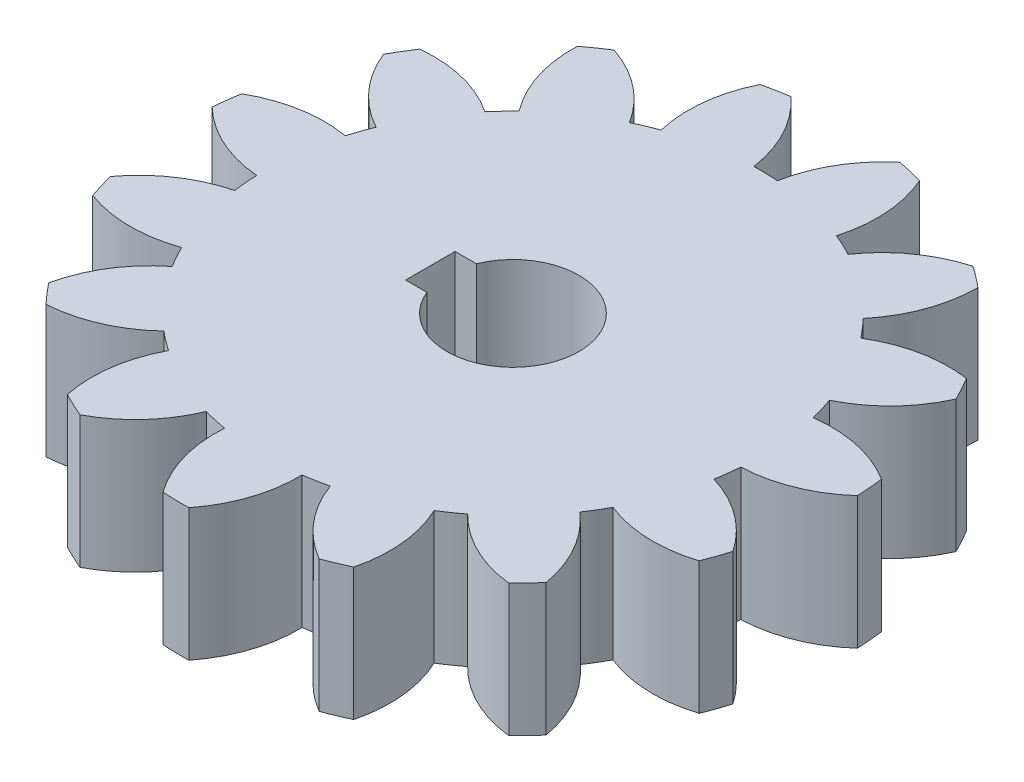
SolidWorks part; units mm, degrees
ref_plane "Front Plane" through (0, 0, 0) normal (0, 0, 1) x (1, 0, 0)
ref_plane "Top Plane" through (0, 0, 0) normal (0, 1, 0) x (1, 0, 0)
ref_plane "Right Plane" through (0, 0, 0) normal (1, 0, 0) x (0, 0, -1)
other "Configuration Table"
sketch "Sketch1" plane through (0, 0, 0) normal (0, 1, 0) x (1, 0, 0)
  line L0 (-43.1275, 149.2664) -> (-24.4163, 51.0325) construction
  line L1 (-42.9568, 58.5325) -> (-49.4163, 58.5325)
  line L2 (-42.9568, 43.5325) -> (-49.4163, 43.5325)
  line L5 (-49.4163, 43.5325) -> (-49.4163, 58.5325)
  line L6 (5.1882, 42.1512) -> (-49.4163, 58.5325) construction
  line L7 (5.1882, 59.9139) -> (-49.4163, 43.5325) construction
  arc A0 (-47.0419, 148.4393) -> (-39.1832, 149.9362) centre (-24.4163, 51.0325) cw
  arc A1 (10.8043, 117.2482) -> (4.1913, 120.3622) centre (-24.4163, 51.0325) ccw
  arc A2 (-47.0419, 148.4393) -> (-50.057, 121.5134) centre (-11.1471, 130.7882) ccw
  arc A3 (-39.1832, 149.9362) -> (-26.4808, 126.0041) centre (-66.0757, 120.3256) cw
  arc A4 (-5.4669, 149.2207) -> (-19.173, 125.849) centre (20.1453, 118.4959) ccw
  arc A5 (2.3213, 147.3918) -> (4.1913, 120.3622) centre (-34.29, 131.2793) cw
  arc A6 (-5.4669, 149.2207) -> (2.3213, 147.3918) centre (-24.4163, 51.0325) cw
  arc A7 (32.8316, 133.0245) -> (10.8043, 117.2482) centre (43.7325, 94.5385) ccw
  arc A8 (39.2025, 128.186) -> (29.917, 102.7326) centre (-0.7971, 128.3576) cw
  arc A9 (32.8316, 133.0245) -> (39.2025, 128.186) centre (-24.4163, 51.0325) cw
  arc A10 (61.2314, 102.6511) -> (34.6916, 97.1981) centre (55.5362, 63.0586) ccw
  arc A11 (65.0835, 95.6396) -> (46.2479, 76.1635) centre (28.6118, 112.0657) cw
  arc A12 (61.2314, 102.6511) -> (65.0835, 95.6396) centre (-24.4163, 51.0325) cw
  arc A13 (74.8219, 63.3524) -> (48.3587, 69.1655) centre (53.5154, 29.4993) ccw
  arc A14 (75.4892, 55.3803) -> (50.3604, 45.2491) centre (48.8517, 85.2207) cw
  arc A15 (74.8219, 63.3524) -> (75.4892, 55.3803) centre (-24.4163, 51.0325) cw
  arc A16 (71.2533, 21.9235) -> (49.4423, 37.9976) centre (38.0195, -0.3367) ccw
  arc A17 (68.6203, 14.3692) -> (41.5433, 15.3347) centre (56.423, 52.4642) cw
  arc A18 (71.2533, 21.9235) -> (68.6203, 14.3692) centre (-24.4163, 51.0325) cw
  arc A19 (51.1425, -14.4722) -> (37.7551, 9.0835) centre (11.7279, -21.2906) ccw
  arc A20 (45.6645, -20.3025) -> (21.3212, -8.4072) centre (50.0163, 19.4601) cw
  arc A21 (51.1425, -14.4722) -> (45.6645, -20.3025) centre (-24.4163, 51.0325) cw
  arc A22 (17.9669, -39.5415) -> (15.3179, -12.5772) centre (-20.8134, -29.7391) ccw
  arc A23 (10.5911, -42.6397) -> (-6.8094, -21.8715) centre (30.7396, -8.0848) cw
  arc A24 (17.9669, -39.5415) -> (10.5911, -42.6397) centre (-24.4163, 51.0325) cw
  arc A25 (-22.5371, -48.9498) -> (-13.9897, -23.2392) centre (-53.9777, -24.2214) ccw
  arc A26 (-30.5353, -48.7801) -> (-37.9843, -22.73) centre (1.926, -25.4077) cw
  arc A27 (-22.5371, -48.9498) -> (-30.5353, -48.7801) centre (-24.4163, 51.0325) cw
  arc A28 (-63.3661, -41.0702) -> (-45.1002, -21.0589) centre (-82.0305, -5.6917) ccw
  arc A29 (-70.6038, -37.662) -> (-66.8132, -10.8343) centre (-31.4425, -29.5135) cw
  arc A30 (-63.3661, -41.0702) -> (-70.6038, -37.662) centre (-24.4163, 51.0325) cw
  arc A31 (-97.4602, -17.2652) -> (-72.6342, -6.4134) centre (-100.1213, 22.6462) ccw
  arc A32 (-102.6859, -11.2078) -> (-88.3113, 11.7588) centre (-63.5961, -19.6921) cw
  arc A33 (-97.4602, -17.2652) -> (-102.6859, -11.2078) centre (-24.4163, 51.0325) cw
  arc A34 (-118.9244, 18.3491) -> (-91.8309, 18.1651) centre (-105.122, 55.8923) ccw
  arc A35 (-121.2346, 26.0083) -> (-98.7614, 41.1426) centre (-88.9751, 2.3582) cw
  arc A36 (-118.9244, 18.3491) -> (-121.2346, 26.0083) centre (-24.4163, 51.0325) cw
  arc A37 (-124.0473, 59.6147) -> (-99.371, 48.4266) centre (-96.168, 88.2982) ccw
  arc A38 (-123.0425, 67.5513) -> (-96.3565, 72.2365) centre (-103.1913, 32.8248) cw
  arc A39 (-124.0473, 59.6147) -> (-123.0425, 67.5513) centre (-24.4163, 51.0325) cw
  arc A40 (-111.9431, 99.3963) -> (-93.9508, 79.1387) centre (-74.8074, 114.2604) ccw
  arc A41 (-107.797, 106.2381) -> (-81.5125, 99.6641) centre (-103.7866, 66.4396) cw
  arc A42 (-111.9431, 99.3963) -> (-107.797, 106.2381) centre (-24.4163, 51.0325) cw
  arc A43 (-84.7047, 130.8154) -> (-76.5074, 104.991) centre (-44.7338, 129.29) ccw
  arc A44 (-78.1343, 135.3793) -> (-56.796, 118.6828) centre (-90.6581, 97.3905) cw
  arc A45 (-84.7047, 130.8154) -> (-78.1343, 135.3793) centre (-24.4163, 51.0325) cw
  arc A46 (-76.5074, 104.991) -> (-81.5125, 99.6641) centre (-24.4163, 51.0325) ccw
  arc A47 (-93.9508, 79.1387) -> (-96.3565, 72.2365) centre (-24.4163, 51.0325) ccw
  arc A48 (-99.371, 48.4266) -> (-98.7614, 41.1426) centre (-24.4163, 51.0325) ccw
  arc A49 (-91.8309, 18.1651) -> (-88.3113, 11.7588) centre (-24.4163, 51.0325) ccw
  arc A50 (-72.6342, -6.4134) -> (-66.8132, -10.8343) centre (-24.4163, 51.0325) ccw
  arc A51 (-45.1002, -21.0589) -> (-37.9843, -22.73) centre (-24.4163, 51.0325) ccw
  arc A52 (15.3179, -12.5772) -> (21.3212, -8.4072) centre (-24.4163, 51.0325) ccw
  arc A53 (-13.9897, -23.2392) -> (-6.8094, -21.8715) centre (-24.4163, 51.0325) ccw
  arc A54 (-19.173, 125.849) -> (-26.4808, 126.0041) centre (-24.4163, 51.0325) ccw
  arc A55 (-50.057, 121.5134) -> (-56.796, 118.6828) centre (-24.4163, 51.0325) ccw
  arc A56 (34.6916, 97.1981) -> (29.917, 102.7326) centre (-24.4163, 51.0325) ccw
  arc A57 (48.3587, 69.1655) -> (46.2479, 76.1635) centre (-24.4163, 51.0325) ccw
  arc A58 (49.4423, 37.9976) -> (50.3604, 45.2491) centre (-24.4163, 51.0325) ccw
  arc A59 (37.7551, 9.0835) -> (41.5433, 15.3347) centre (-24.4163, 51.0325) ccw
  arc A60 (-42.9568, 43.5325) -> (-42.9568, 58.5325) centre (-24.4163, 51.0325) ccw
  dimension "D1" = 100
  dimension "D4" = 40
  dimension "D5" = 40
  dimension "D6" = 40
  dimension "D2" = 4
  dimension "D3" = 12
  dimension "D7" = 15
  dimension "D8" = 25
extrude "Boss-Extrude1" add sketch "Sketch1" along normal blind 40
